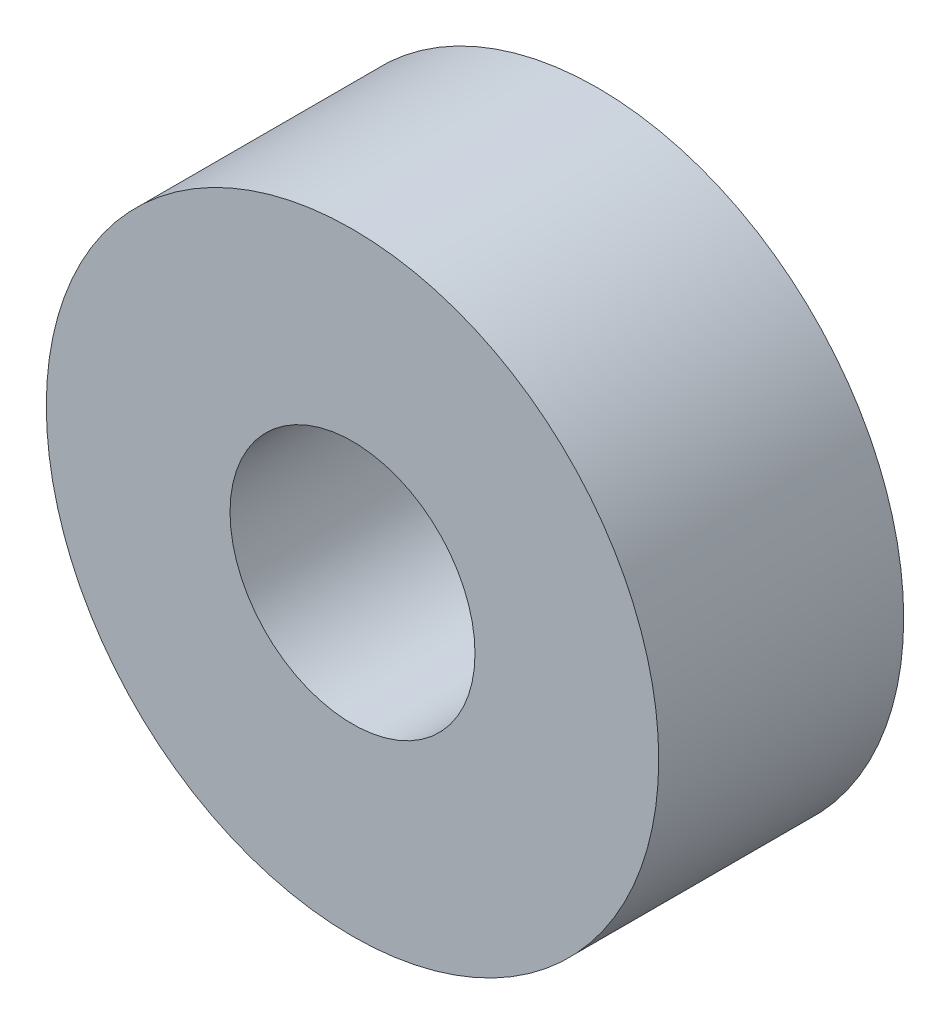
from build123d import *

# Parameters (mm, degrees)
SKETCH1_R           = 2.5
SKETCH1_R_2         = 1
BOSS_EXTRUDE1_DEPTH = 2


with BuildPart() as part:
    # Sketch1 → Boss-Extrude1 (new body)
    with BuildSketch(Plane.XY):
        with Locations((-220.5, 0)):
            Circle(SKETCH1_R)
        with Locations((-220.5, 0)):
            Circle(SKETCH1_R_2, mode=Mode.SUBTRACT)
    extrude(amount=BOSS_EXTRUDE1_DEPTH)


solid = part.part
